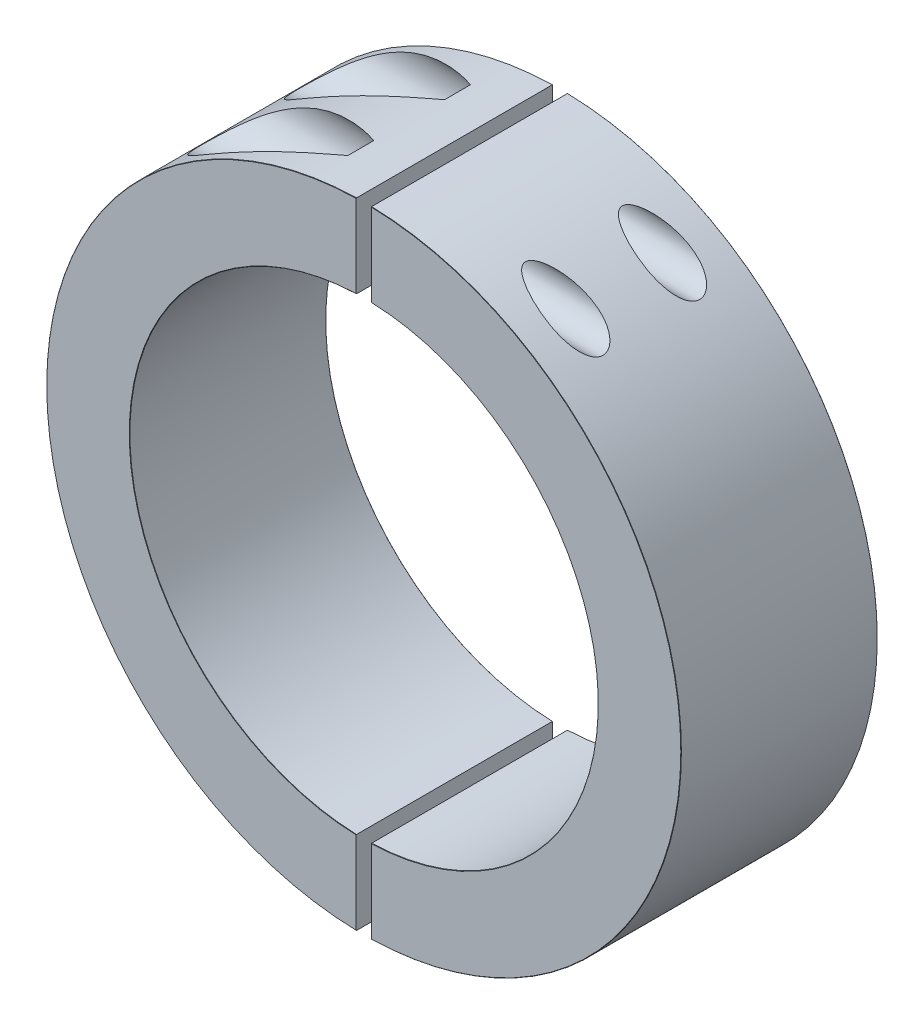
from build123d import *

# Parameters (mm, degrees)
SKETCH1_R                   = 105
SKETCH1_R_2                 = 77.5
BOSS_EXTRUDE1_DEPTH         = 65
CHAMFER1_SIZE               = 0.1
SKETCH2_W                   = 5
SKETCH2_H                   = 290.90208271
CUT_EXTRUDE1_DEPTH          = 163.095650774
CUT_EXTRUDE2_START          = -15
SKETCH3_R                   = 13
CUT_EXTRUDE2_DEPTH          = 149.707055437
SKETCH4_R                   = 8.5
CUT_EXTRUDE3_DEPTH          = 16
SKETCH7_W                   = 7
SKETCH7_H                   = 102.5
M16_TAPPED_HOLE1_AT_2_COUNT = 2
M16_TAPPED_HOLE1_AT_2_PITCH = 32
MIRROR1_COPY_1_SKETCH_W     = 7
MIRROR1_COPY_1_SKETCH_H     = 102.5


with BuildPart() as part:
    # Sketch1 → Boss-Extrude1 (new body)
    with BuildSketch(Plane.XY):
        Circle(SKETCH1_R)
        Circle(SKETCH1_R_2, mode=Mode.SUBTRACT)
    extrude(amount=BOSS_EXTRUDE1_DEPTH)

    # Chamfer1
    chamfer1_edges = [part.edges().sort_by_distance(p)[0] for p in [
        (-105, 0, 0),
        (-105, 0, 65),
        (-77.5, 0, 0),
        (-77.5, 0, 65),
    ]]
    chamfer(chamfer1_edges, length=CHAMFER1_SIZE)

    # Sketch2 → Cut-Extrude1 (cut, through all)
    with BuildSketch(Plane(origin=(0, 0, 0), x_dir=(-1, 0, 0), z_dir=(0, 0, -1))):
        Rectangle(SKETCH2_W, SKETCH2_H)
    extrude(amount=-CUT_EXTRUDE1_DEPTH, mode=Mode.SUBTRACT)


with BuildPart() as cut_extrude1_piece_1:
    # of the separate pieces the step leaves, piece 1, a body of its own (cut_extrude1_pieces)
    add(part.part.solids().sort_by_distance((2.5, -104.970233876, 0.1))[0])

    # Sketch7 → M16 Tapped Hole1 (revolve, cut)
    with BuildSketch(Plane(origin=(2.5, 91.25, 48.5), x_dir=(0, 0, 1), z_dir=(0, 1, 0))):
        with Locations((3.5, 51.25)):
            Rectangle(SKETCH7_W, SKETCH7_H)
    m16_tapped_hole1 = revolve(axis=Axis((-3.85, 91.25, 48.5), (1, 0, 0)), mode=Mode.SUBTRACT)

    # M16 Tapped Hole1 at 2: M16 Tapped Hole1 ×2
    with Locations(*[(0, 0, -i * M16_TAPPED_HOLE1_AT_2_PITCH) for i in range(1, M16_TAPPED_HOLE1_AT_2_COUNT)]):
        add(m16_tapped_hole1, mode=Mode.SUBTRACT)

    # Mirror1: M16 Tapped Hole1 across plane
    add(m16_tapped_hole1.mirror(Plane.ZX), mode=Mode.SUBTRACT)

    # Mirror1 copy 1 sketch → Mirror1 copy 1 (revolve, cut)
    with BuildSketch(Plane(origin=(2.5, -91.25, 16.5), x_dir=(0, 0, 1), z_dir=(0, -1, 0))):
        with Locations((3.5, -51.25)):
            Rectangle(MIRROR1_COPY_1_SKETCH_W, MIRROR1_COPY_1_SKETCH_H)
    revolve(axis=Axis((-3.85, -91.25, 16.5), (-1, 0, 0)), mode=Mode.SUBTRACT)


with BuildPart() as cut_extrude1_piece_2:
    # of the separate pieces the step leaves, piece 2, a body of its own (cut_extrude1_pieces)
    add(part.part.solids().sort_by_distance((-2.5, 104.970233876, 0.1))[0])

    # Sketch3 → Cut-Extrude2 (cut, through all)
    with BuildSketch(Plane(origin=(-2.5, 0, 0), x_dir=(0, 0, -1), z_dir=(1, 0, 0)).offset(CUT_EXTRUDE2_START)):
        with Locations((-48.5, 91.25)):
            Circle(SKETCH3_R)
        with Locations((-16.5, 91.25)):
            Circle(SKETCH3_R)
    cut_extrude2 = extrude(amount=-CUT_EXTRUDE2_DEPTH, mode=Mode.SUBTRACT)

    # Sketch4 → Cut-Extrude3 (cut)
    with BuildSketch(Plane.ZY.offset(17.5)):
        with Locations(Location((48.5, 91.25, 0), (0, 0, 270))):
            Circle(SKETCH4_R)
        with Locations(Location((16.5, 91.25, 0), (0, 0, 270))):
            Circle(SKETCH4_R)
    cut_extrude3 = extrude(amount=-CUT_EXTRUDE3_DEPTH, mode=Mode.SUBTRACT)

    # Mirror2: Cut-Extrude2 across plane
    add(cut_extrude2.mirror(Plane.ZX), mode=Mode.SUBTRACT)

    # Mirror3: Cut-Extrude3 across plane
    add(cut_extrude3.mirror(Plane.ZX), mode=Mode.SUBTRACT)


solid = Compound([cut_extrude1_piece_1.part, cut_extrude1_piece_2.part])
